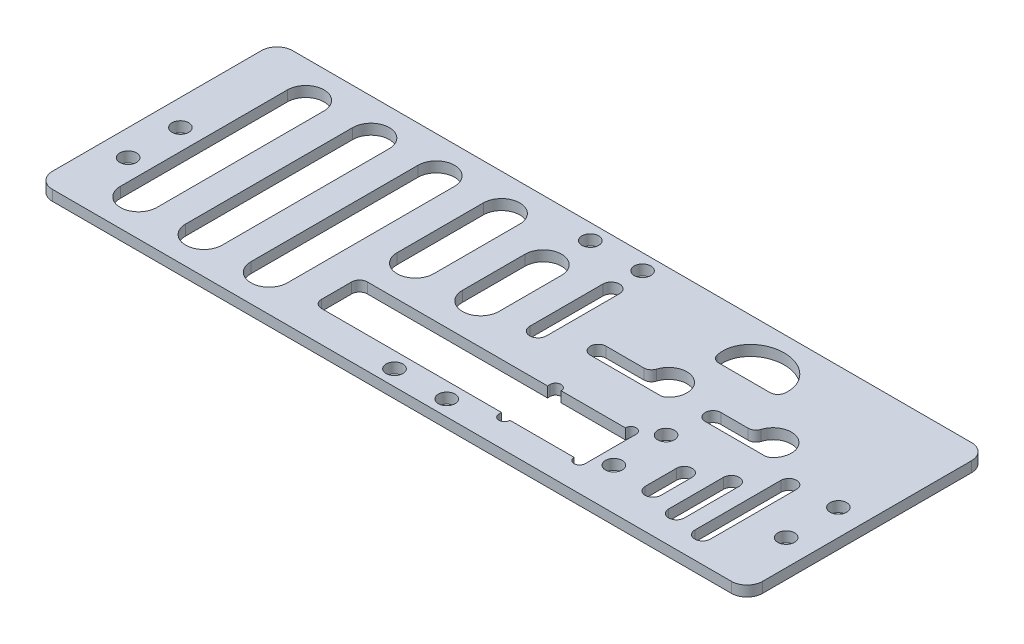
from build123d import *

# Parameters (mm, degrees)
SKETCH1_W              = 136
SKETCH1_H              = 46
SKETCH1_R              = 1.6
BOSS_EXTRUDE1_DEPTH    = 2
CUT_EXTRUDE1_DEPTH     = 72.812255222
R1_5_CUTOUT_FILLET_R   = 1.5
R3_OUTER_EDGE_FILLET_R = 3


with BuildPart() as part:
    # Sketch1 → Boss-Extrude1 (new body)
    with BuildSketch(Plane(origin=(0, 0, 0), x_dir=(1, 0, 0), z_dir=(0, 1, 0))):
        Rectangle(SKETCH1_W, SKETCH1_H)
        with Locations(Location((-63, -0.5, 0), (0, 0, 270))):
            Circle(SKETCH1_R, mode=Mode.SUBTRACT)
        with Locations(Location((-63, -10.5, 0), (0, 0, 270))):
            Circle(SKETCH1_R, mode=Mode.SUBTRACT)
        with Locations(Location((-2.5, -20, 0), (0, 0, 270))):
            Circle(SKETCH1_R, mode=Mode.SUBTRACT)
        with Locations(Location((7.5, -20, 0), (0, 0, 270))):
            Circle(SKETCH1_R, mode=Mode.SUBTRACT)
        with Locations(Location((63, -10.5, 0), (0, 0, 90))):
            Circle(SKETCH1_R, mode=Mode.SUBTRACT)
        with Locations(Location((63, -0.5, 0), (0, 0, 90))):
            Circle(SKETCH1_R, mode=Mode.SUBTRACT)
        with Locations(Location((5, 20, 0), (0, 0, 270))):
            Circle(SKETCH1_R, mode=Mode.SUBTRACT)
        with Locations(Location((-5, 20, 0), (0, 0, 270))):
            Circle(SKETCH1_R, mode=Mode.SUBTRACT)
        with Locations(Location((34.5, -5, 0), (0, 0, 270))):
            Circle(SKETCH1_R, mode=Mode.SUBTRACT)
        with Locations(Location((34.5, -15, 0), (0, 0, 270))):
            Circle(SKETCH1_R, mode=Mode.SUBTRACT)
    extrude(amount=BOSS_EXTRUDE1_DEPTH)

    # Sketch2 → Cut-Extrude1 (cut, through all)
    with BuildSketch(Plane(origin=(0, 2, 0), x_dir=(1, 0, 0), z_dir=(0, 1, 0))):
        with BuildLine():
            Line((-52, 16), (-52, -16))
            ThreePointArc((-52, -16), (-55.5, -19.5), (-59, -16))
            Line((-59, -16), (-59, 16))
            ThreePointArc((-59, 16), (-55.5, 19.5), (-52, 16))
        make_face()
        with BuildLine():
            Line((17.1, -7.7), (29.4, -7.7))
            ThreePointArc((29.4, -7.7), (30.45, -6.65), (31.5, -7.7))
            Line((31.5, -7.7), (31.5, -17.5))
            ThreePointArc((31.5, -17.5), (30.45, -18.55), (29.4, -17.5))
            Line((29.4, -17.5), (17.1, -17.5))
            ThreePointArc((17.1, -17.5), (16.05, -18.55), (15, -17.5))
            Line((15, -17.5), (15, -17))
            Line((15, -17), (-21, -17))
            Line((-21, -17), (-21, -8.2))
            Line((-21, -8.2), (15, -8.2))
            Line((15, -8.2), (15, -7.7))
            ThreePointArc((15, -7.7), (16.05, -6.65), (17.1, -7.7))
        make_face()
        with BuildLine():
            Line((-39.5, 16), (-39.5, -16))
            ThreePointArc((-39.5, -16), (-43, -19.5), (-46.5, -16))
            Line((-46.5, -16), (-46.5, 16))
            ThreePointArc((-46.5, 16), (-43, 19.5), (-39.5, 16))
        make_face()
        with BuildLine():
            Line((-27, 16), (-27, -16))
            ThreePointArc((-27, -16), (-30.5, -19.5), (-34, -16))
            Line((-34, -16), (-34, 16))
            ThreePointArc((-34, 16), (-30.5, 19.5), (-27, 16))
        make_face()
        with BuildLine():
            Line((-2, 11.5), (-2, -0.5))
            ThreePointArc((-2, -0.5), (-5.5, -4), (-9, -0.5))
            Line((-9, -0.5), (-9, 11.5))
            ThreePointArc((-9, 11.5), (-5.5, 15), (-2, 11.5))
        make_face()
        with BuildLine():
            Line((42.5, 4), (36, 4))
            ThreePointArc((36, 4), (34.5, 2.5), (36, 1))
            Line((36, 1), (47.802775638, 1))
            ThreePointArc((47.802775638, 1), (47.723410176, 7.046285831), (42.5, 4))
        make_face()
        with BuildLine():
            Line((41, -15.5), (41, -9.5))
            ThreePointArc((41, -9.5), (42.5, -8), (44, -9.5))
            Line((44, -9.5), (44, -15.5))
            ThreePointArc((44, -15.5), (42.5, -17), (41, -15.5))
        make_face()
        with BuildLine():
            Line((47, -17), (47, -6.5))
            ThreePointArc((47, -6.5), (48.5, -5), (50, -6.5))
            Line((50, -6.5), (50, -17))
            ThreePointArc((50, -17), (48.5, -18.5), (47, -17))
        make_face()
        with BuildLine():
            Line((53, -18), (53, -1.5))
            ThreePointArc((53, -1.5), (54.5, 0), (56, -1.5))
            Line((56, -1.5), (56, -18))
            ThreePointArc((56, -18), (54.5, -19.5), (53, -18))
        make_face()
        with BuildLine():
            Line((22.5, 4), (14, 4))
            ThreePointArc((14, 4), (12.5, 2.5), (14, 1))
            Line((14, 1), (27.802775638, 1))
            ThreePointArc((27.802775638, 1), (27.723410176, 7.046285831), (22.5, 4))
        make_face()
        with BuildLine():
            Line((38.555359619, 12), (26.555359619, 12))
            add(Edge.make_bspline(
                [(38.555359619, 12), (41.784518916, 19.940569638), (32.181153285, 19.940569638), (22.577787653, 19.940569638), (26.555359619, 12)],
                knots=[6.095299784, 6.095299784, 6.095299784, 8.050729179, 8.050729179, 10.006158574, 10.006158574, 10.006158574], degree=2, weights=[1, 0.558919028, 1, 0.558919028, 1]))
        make_face()
        with BuildLine():
            Line((3.4, 0), (3.4, 14))
            ThreePointArc((3.4, 14), (5, 15.6), (6.6, 14))
            Line((6.6, 14), (6.6, 0))
            ThreePointArc((6.6, 0), (5, -1.6), (3.4, 0))
        make_face()
        with BuildLine():
            Line((-21.5, -0.5), (-21.5, 16))
            ThreePointArc((-21.5, 16), (-18, 19.5), (-14.5, 16))
            Line((-14.5, 16), (-14.5, -0.5))
            ThreePointArc((-14.5, -0.5), (-18, -4), (-21.5, -0.5))
        make_face()
    extrude(amount=-CUT_EXTRUDE1_DEPTH, mode=Mode.SUBTRACT)

    # R1.5 cutout fillet
    r1_5_cutout_fillet_edges = [part.edges().sort_by_distance(p)[0] for p in [
        (-21, 1, 8.2),
        (-21, 1, 17),
        (38.555359619, 1, -12),
        (26.555359619, 1, -12),
        (22.5, 1, -4),
        (27.802775638, 1, -1),
        (42.5, 1, -4),
        (47.802775638, 1, -1),
    ]]
    fillet(r1_5_cutout_fillet_edges, radius=R1_5_CUTOUT_FILLET_R)

    # R3 outer edge fillet
    r3_outer_edge_fillet_edges = [part.edges().sort_by_distance(p)[0] for p in [
        (-68, 1, -23),
        (68, 1, -23),
        (68, 1, 23),
        (-68, 1, 23),
    ]]
    fillet(r3_outer_edge_fillet_edges, radius=R3_OUTER_EDGE_FILLET_R)


solid = part.part
